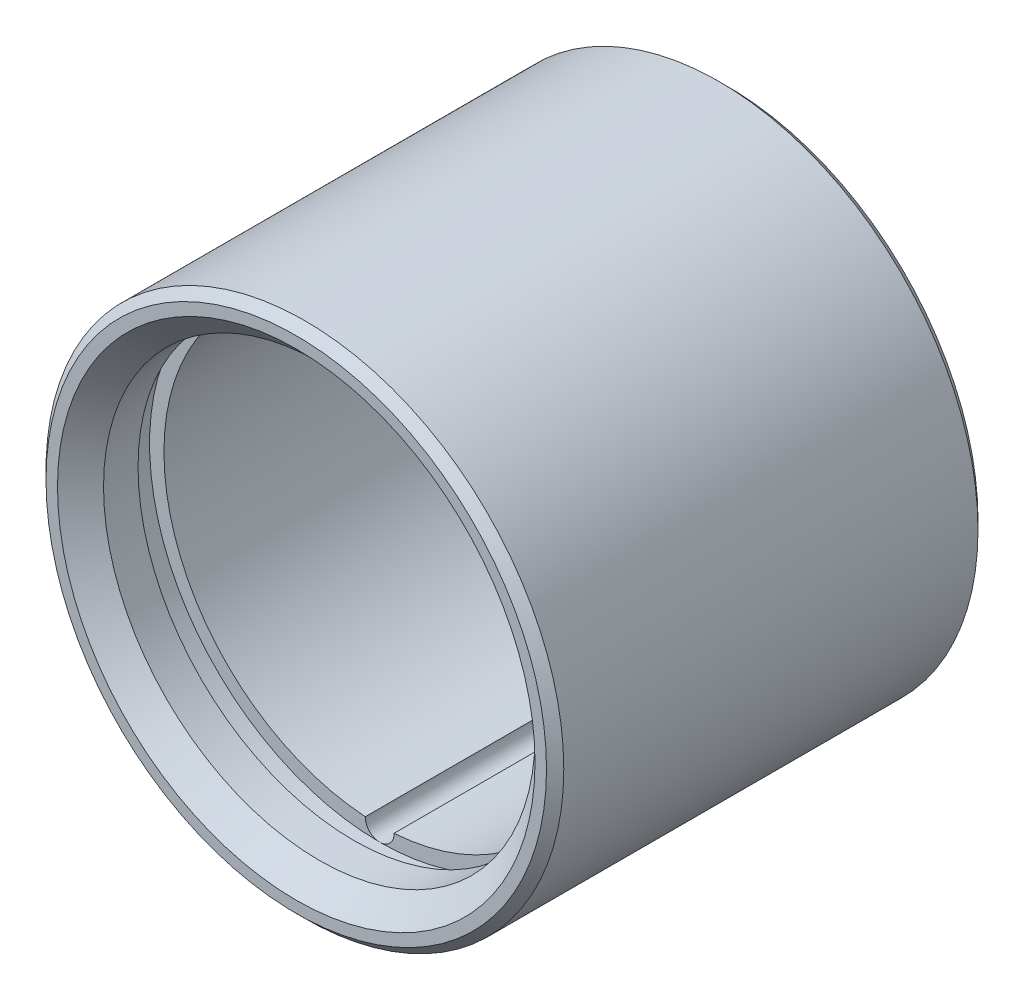
from build123d import *

# Parameters (mm, degrees)
SKETCH1_R           = 45
SKETCH1_R_2         = 37.5
BOSS_EXTRUDE1_DEPTH = 37.5
CUT_EXTRUDE1_START  = -4.5
SKETCH2_R           = 40
SKETCH2_R_2         = 37.5
CUT_EXTRUDE1_DEPTH  = 4.5
CHAMFERC1_5_SIZE    = 1.5
CHAMFERC4_SIZE      = 4
CUT_EXTRUDE2_DEPTH  = 91.967026993


with BuildPart() as part:
    # Sketch1 → Boss-Extrude1 (new, symmetric)
    with BuildSketch(Plane.XY):
        Circle(SKETCH1_R)
        Circle(SKETCH1_R_2, mode=Mode.SUBTRACT)
    extrude(amount=BOSS_EXTRUDE1_DEPTH, both=True)

    # Sketch2 → Cut-Extrude1 (cut)
    with BuildSketch(Plane.XY.offset(27.5).offset(CUT_EXTRUDE1_START)):
        Circle(SKETCH2_R)
        Circle(SKETCH2_R_2, mode=Mode.SUBTRACT)
    extrude(amount=CUT_EXTRUDE1_DEPTH, mode=Mode.SUBTRACT)

    # ChamferC1.5
    chamferc1_5_edges = [part.edges().sort_by_distance(p)[0] for p in [
        (-45, 0, -37.5),
        (-45, 0, 37.5),
        (-37.5, 0, -37.5),
    ]]
    chamfer(chamferc1_5_edges, length=CHAMFERC1_5_SIZE)

    # ChamferC4
    chamferc4_edges = [part.edges().sort_by_distance(p)[0] for p in [
        (-37.5, 0, 37.5),
    ]]
    chamfer(chamferc4_edges, length=CHAMFERC4_SIZE)

    # Sketch3 → Cut-Extrude2 (cut, through all)
    with BuildSketch(Plane.XY.offset(27.5)):
        with BuildLine():
            ThreePointArc((2.498610725, 37.416666667), (0, 37.5), (-2.498610725, 37.416666667))
            ThreePointArc((-2.498610725, 37.416666667), (0, 40), (2.498610725, 37.416666667))
        make_face()
        with BuildLine():
            ThreePointArc((-2.498610725, -37.416666667), (0, -40), (2.498610725, -37.416666667))
            ThreePointArc((2.498610725, -37.416666667), (0, -37.5), (-2.498610725, -37.416666667))
        make_face()
    extrude(amount=-CUT_EXTRUDE2_DEPTH, mode=Mode.SUBTRACT)


solid = part.part
